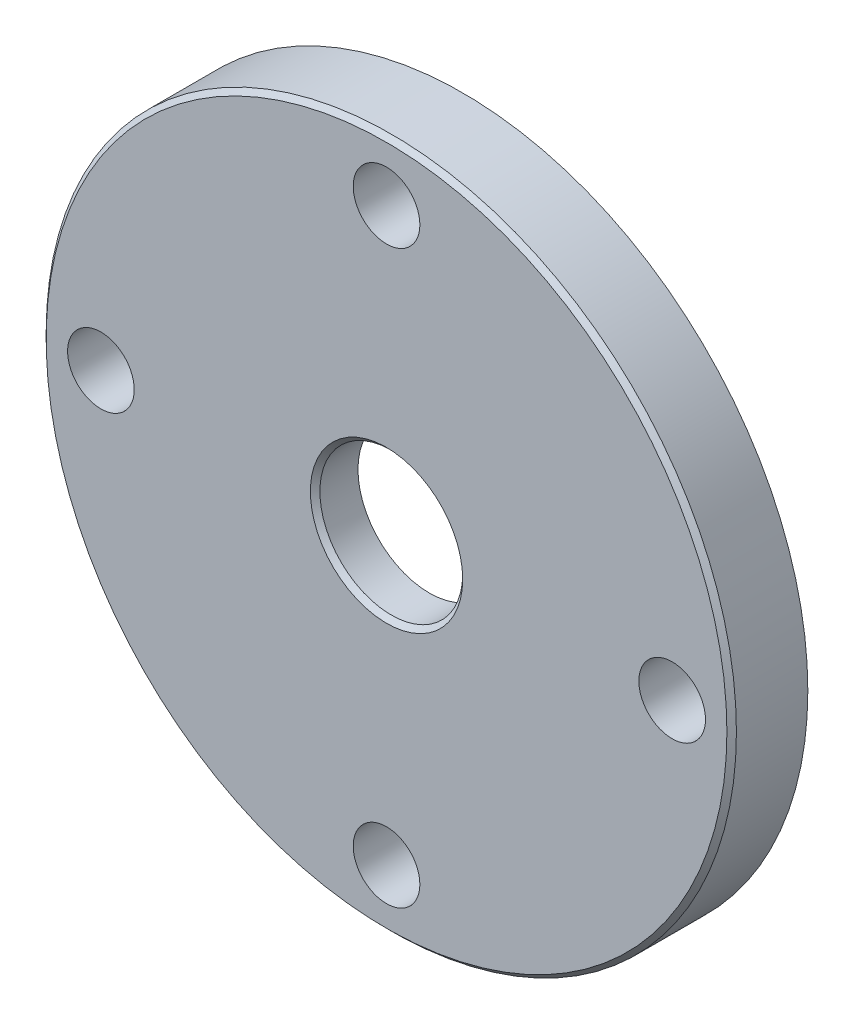
from build123d import *

# Parameters (mm, degrees)
SKETCH_1_R          = 72.5
EXTRUDE_1_DEPTH     = 16
SKETCH_2_R          = 7
CUT_EXTRUDE_1_DEPTH = 104.771383339
SKETCH_3_R          = 46
CUT_EXTRUDE_2_DEPTH = 7
SKETCH_4_R          = 15
CUT_EXTRUDE_3_DEPTH = 104.771383339
CHAMFER_1_SIZE      = 1


with BuildPart() as part:
    # 草图1 → 凸台-拉伸1 (new body)
    with BuildSketch(Plane.XY):
        Circle(SKETCH_1_R)
    extrude(amount=EXTRUDE_1_DEPTH)

    # 草图2 → 切除-拉伸1 (cut, through all)
    with BuildSketch(Plane.XY.offset(16)):
        with Locations((0, 60)):
            Circle(SKETCH_2_R)
        with Locations((60, 0)):
            Circle(SKETCH_2_R)
        with Locations((0, -60)):
            Circle(SKETCH_2_R)
        with Locations((-60, 0)):
            Circle(SKETCH_2_R)
    extrude(amount=-CUT_EXTRUDE_1_DEPTH, mode=Mode.SUBTRACT)

    # 草图3 → 切除-拉伸2 (cut)
    with BuildSketch(Plane(origin=(0, 0, 0), x_dir=(-1, 0, 0), z_dir=(0, 0, -1))):
        Circle(SKETCH_3_R)
    extrude(amount=-CUT_EXTRUDE_2_DEPTH, mode=Mode.SUBTRACT)

    # 草图4 → 切除-拉伸3 (cut, through all)
    with BuildSketch(Plane.XY.offset(16)):
        Circle(SKETCH_4_R)
    extrude(amount=-CUT_EXTRUDE_3_DEPTH, mode=Mode.SUBTRACT)

    # 倒角1
    chamfer_1_edges = [part.edges().sort_by_distance(p)[0] for p in [
        (46, 0, 0),
        (-15, 0, 16),
        (-72.5, 0, 16),
    ]]
    chamfer(chamfer_1_edges, length=CHAMFER_1_SIZE)


solid = part.part
